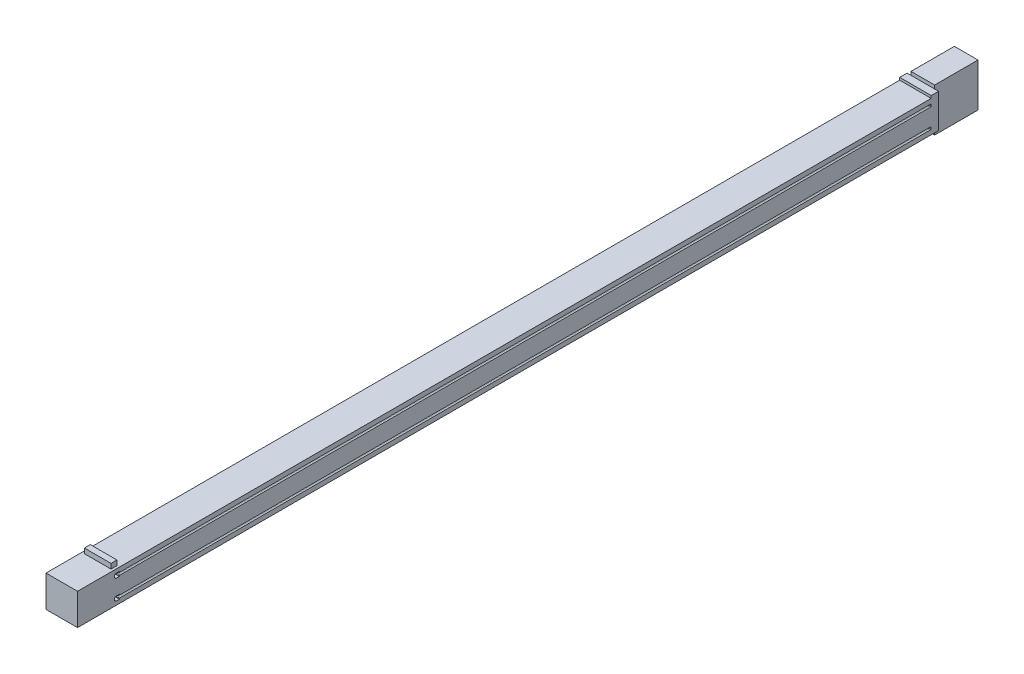
from build123d import *

# Parameters (mm, degrees)
EXTRUDE_642_DEPTH   = 1648
SKETCH_2_W          = 64
SKETCH_2_H          = 64
EXTRUDE_1_DEPTH     = 85
SKETCH_4_W          = 54
SKETCH_4_H          = 12
EXTRUDE_2_DEPTH     = 10
CUT_EXTRUDE_1_DEPTH = 10
SKETCH_6_W          = 64
SKETCH_6_H          = 69
EXTRUDE_3_DEPTH     = 15
SKETCH_7_W          = 48
SKETCH_7_H          = 88
EXTRUDE_4_DEPTH     = 88
SKETCH_8_R          = 36.5
CUT_EXTRUDE_2_DEPTH = 3
SKETCH_9_R          = 8
EXTRUDE_5_DEPTH     = 19


with BuildPart() as part:
    # 草图1 → Extrude 642 (new body)
    with BuildSketch(Plane.XY):
        Polygon((9.931917842, 6.925864063), (9.931917842, 41.925864063), (12.931917842, 41.925864063), (12.931917842, 40.425864063), (16.931917842, 40.425864063), (16.931917842, 48.425864063), (12.931917842, 48.425864063), (12.931917842, 46.925864063), (9.931917842, 46.925864063), (9.931917842, 56.425864063), (73.931917842, 56.425864063), (73.931917842, 46.925864063), (70.931917842, 46.925864063), (70.931917842, 48.425864063), (66.931917842, 48.425864063), (66.931917842, 40.425864063), (70.931917842, 40.425864063), (70.931917842, 41.925864063), (73.931917842, 41.925864063), (73.931917842, 6.925864063), (70.931917842, 6.925864063), (70.931917842, 8.425864063), (66.931917842, 8.425864063), (66.931917842, 0.425864063), (70.931917842, 0.425864063), (70.931917842, 1.925864063), (73.931917842, 1.925864063), (73.931917842, -7.574135937), (9.931917842, -7.574135937), (9.931917842, 1.925864063), (12.931917842, 1.925864063), (12.931917842, 0.425864063), (16.931917842, 0.425864063), (16.931917842, 8.425864063), (12.931917842, 8.425864063), (12.931917842, 6.925864063), align=None)
    extrude(amount=-EXTRUDE_642_DEPTH)

    # 草图2 → 凸台-拉伸1 (add)
    with BuildSketch(Plane.XY):
        with Locations((41.931917842, 24.425864063)):
            Rectangle(SKETCH_2_W, SKETCH_2_H)
    extrude(amount=EXTRUDE_1_DEPTH)

    # 草图4 → 凸台-拉伸2 (add)
    with BuildSketch(Plane(origin=(0, 56.425864063, 0), x_dir=(-1, 0, 0), z_dir=(0, 1, 0))):
        with Locations((-41.931917842, 6)):
            Rectangle(SKETCH_4_W, SKETCH_4_H)
    extrude(amount=EXTRUDE_2_DEPTH)

    # 草图5 → 切除-拉伸1 (cut)
    with BuildSketch(Plane(origin=(73.931917842, 0, 0), x_dir=(0, 0, -1), z_dir=(1, 0, 0))):
        with BuildLine():
            Line((0, 48.925864063), (-6, 48.925864063))
            ThreePointArc((-6, 48.925864063), (-8.828427125, 47.754291188), (-10, 44.925864063))
            Line((-10, 44.925864063), (-10, 43.925864063))
            ThreePointArc((-10, 43.925864063), (-8.828427125, 41.097436938), (-6, 39.925864063))
            Line((-6, 39.925864063), (0, 39.925864063))
            Line((0, 39.925864063), (0, 48.925864063))
        make_face()
        with BuildLine():
            Line((0, 8.925864063), (-6, 8.925864063))
            ThreePointArc((-6, 8.925864063), (-8.828427125, 7.754291188), (-10, 4.925864063))
            Line((-10, 4.925864063), (-10, 3.925864063))
            ThreePointArc((-10, 3.925864063), (-8.828427125, 1.097436938), (-6, -0.074135937))
            Line((-6, -0.074135937), (0, -0.074135937))
            Line((0, -0.074135937), (0, 8.925864063))
        make_face()
    cut_extrude_1 = extrude(amount=-CUT_EXTRUDE_1_DEPTH, mode=Mode.SUBTRACT)

    # 镜向1: 切除-拉伸1 across plane
    add(cut_extrude_1.mirror(Plane.ZY.offset(-41.931917842)), mode=Mode.SUBTRACT)

    # 草图6 → 凸台-拉伸3 (add)
    with BuildSketch(Plane(origin=(0, 0, -1648), x_dir=(-1, 0, 0), z_dir=(0, 0, -1))):
        with Locations((-41.931917842, 26.925864063)):
            Rectangle(SKETCH_6_W, SKETCH_6_H)
    extrude(amount=EXTRUDE_3_DEPTH)

    # 草图7 → 凸台-拉伸4 (add)
    with BuildSketch(Plane(origin=(0, 0, -1663), x_dir=(-1, 0, 0), z_dir=(0, 0, -1))):
        with Locations((-41.931917842, 24.425864063)):
            Rectangle(SKETCH_7_W, SKETCH_7_H)
    extrude(amount=EXTRUDE_4_DEPTH)

    # 草图8 → 切除-拉伸2 (cut)
    with BuildSketch(Plane.ZY.offset(-17.931917842)):
        with Locations((-1707, 24.425864063)):
            Circle(SKETCH_8_R)
    extrude(amount=-CUT_EXTRUDE_2_DEPTH, mode=Mode.SUBTRACT)

    # 草图9 → 凸台-拉伸5 (add)
    with BuildSketch(Plane.ZY.offset(-20.931917842)):
        with Locations((-1707, 24.425864063)):
            Circle(SKETCH_9_R)
    extrude(amount=EXTRUDE_5_DEPTH)


solid = part.part
